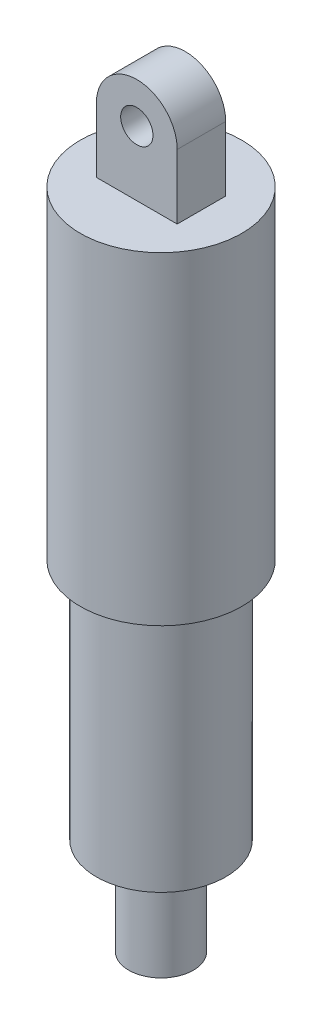
SolidWorks part; units mm, degrees
ref_plane "Front Plane" through (0, 0, 0) normal (0, 0, 1) x (1, 0, 0)
ref_plane "Top Plane" through (0, 0, 0) normal (0, 1, 0) x (1, 0, 0)
ref_plane "Right Plane" through (0, 0, 0) normal (1, 0, 0) x (0, 0, -1)
sketch "Sketch1" plane through (0, 0, 0) normal (0, 0, 1) x (1, 0, 0)
  line L0 (0, 0) -> (0, 410)
  line L1 (0, 410) -> (50, 410)
  line L2 (50, 410) -> (50, 210)
  line L3 (50, 210) -> (40, 210)
  line L4 (40, 210) -> (40, 60)
  line L5 (40, 60) -> (20, 60)
  line L6 (20, 60) -> (20, 0)
  line L7 (20, 0) -> (0, 0)
  dimension "D1" = 20
  dimension "D2" = 60
  dimension "D3" = 40
  dimension "D4" = 50
  dimension "D5" = 150
  dimension "D6" = 200
revolve "Revolve1" add sketch "Sketch1" angle 360 about L0
sketch "Sketch2" plane through (0, 0, 0) normal (0, 0, 1) x (1, 0, 0)
  line L0 (50, 410) -> (-50, 410) construction
  line L1 (-25, 450) -> (-25, 410)
  line L2 (-25, 410) -> (25, 410)
  line L3 (25, 410) -> (25, 450)
  circle A0 centre (0, 450) radius 10
  arc A1 (25, 450) -> (-25, 450) centre (0, 450) ccw
  dimension "D1" = 20
  dimension "D2" = 50
  dimension "D3" = 40
extrude "Boss-Extrude1" add sketch "Sketch2" along normal mid plane 30
